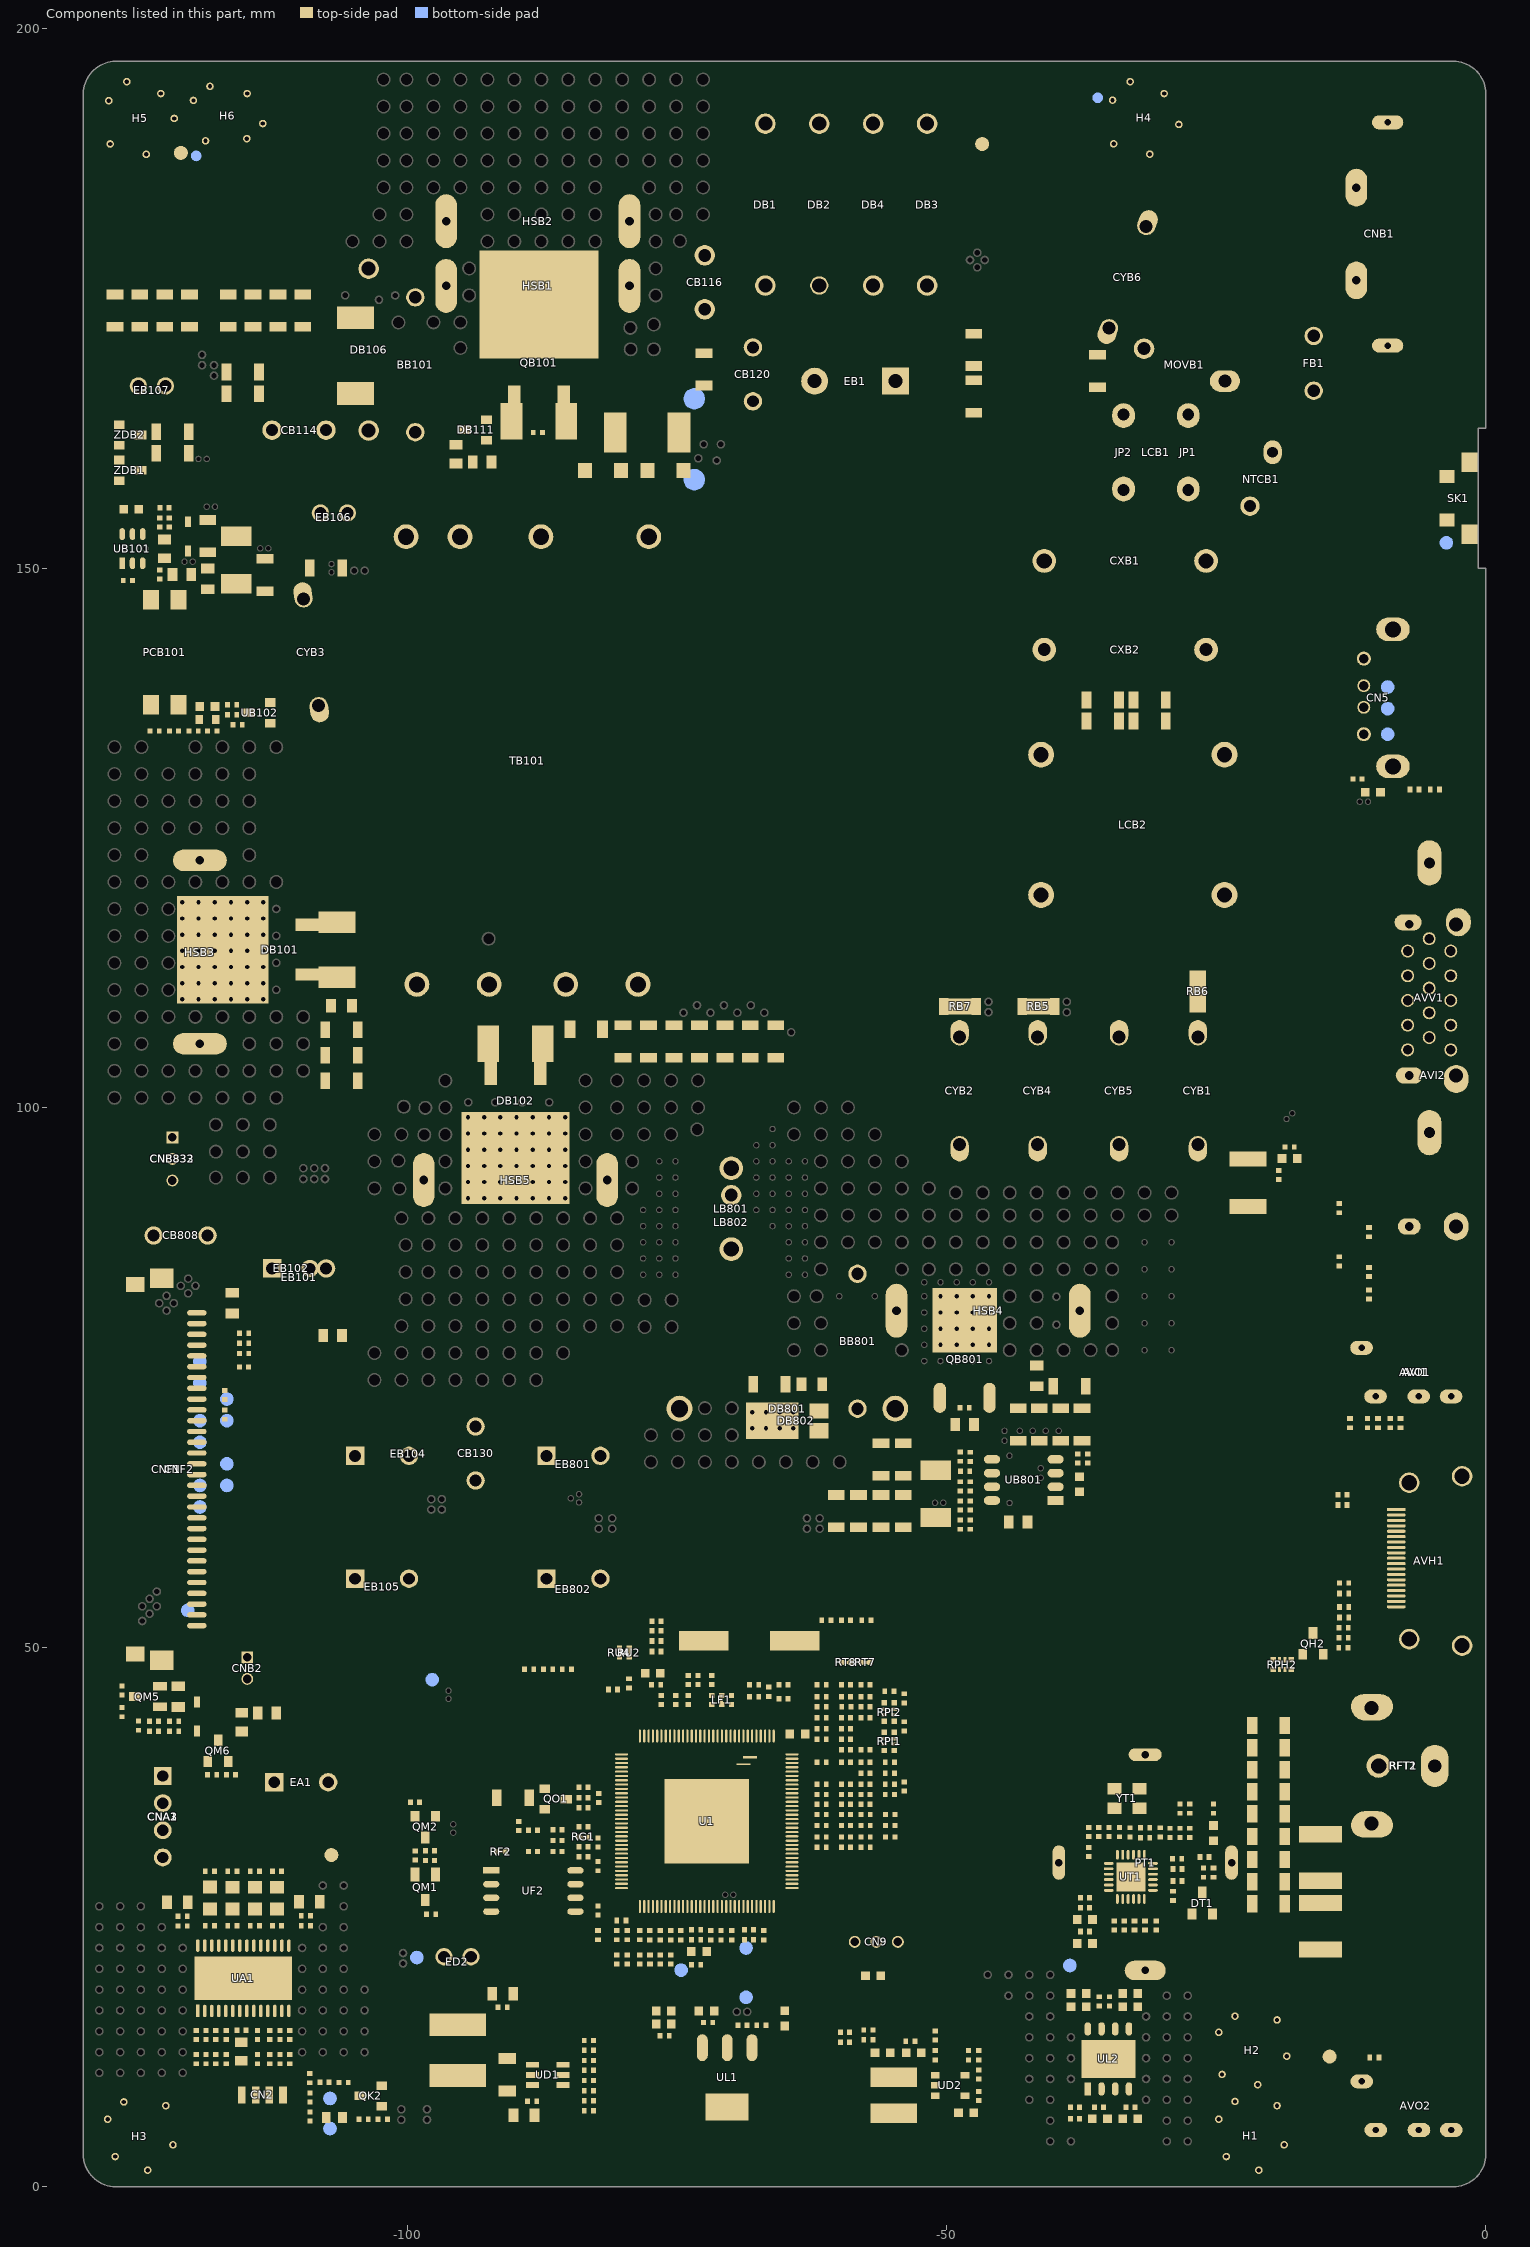
[diagram p0: the components of this part, seen from the top]
# Altium PCB MISC84438.PcbDoc (part 14 of 15)
Units mm, origin at the board's own origin, x right, y up, seen from the top; angles counter-clockwise.
Board outline 130 x 197 mm, 2 copper layers (TopLayer, BottomLayer), stack 1.571 mm thick; 574 components, 314 nets, 2636 pads, 811 vias.

## Other copper
TopLayer:
  drawing of 201 lines, arcs and shapes, not listed
  text "TopLayer" at 176.584,29.998 h1.52
  text ".GTL" at 186.985,29.889 h1.52
BottomLayer:
  rectangle net GND: -121.006,187.35 -118.212,189.408
  rectangle net GND: -48.768,41.034 -48.539,41.669
  rectangle net GND: -7.645,96.266 -3.2,98.806
  rectangle net GND: -2.54,116.18 -0.965,118.923
  rectangle net GND: -2.75,100.736 -1.219,103
  rectangle net GND: -4.661,117 -2.75,119.418
  rectangle net GND: -10.02,129.451 -7.493,131.496
  rectangle net GND: -7.887,121.539 -3.2,123.952
  rectangle net GND: -4.534,101.994 -0.991,103.746
  rectangle: 172.367,23.897 175.674,25.897
  rectangle net GND: -97.155,42.037 -96.862,46.152
  rectangle net GND: -4.978,116.053 -4.521,116.688
  pour cut-out: -35.8,42.2 -20.9,42.2 -20.8,42.1 -20.8,41.529 -35.129,41.529
  pour cut-out: -90.2,54.291 -90.2,58.3 -88.5,60 -87.9,60 -87.9,56.827 -87.073,56
  region net N-1: -14.6,186.4 -14,187 -12.4,187 -12.4,183.6 -14,183.6 -14.6,184.2
  region net D_QB101: -102.502,196.456 -71.349,196.456 -70.866,195.974 -70.866,177.902 -71.526,177.241 -73.707,177.241 -76.429,174.519 -76.429,167.107 -78.461,165.075 -90.634,165.075 -96.679,171.12 -108.814,171.12 -110.541,172.847 -110.541,176.835 -102.819,184.556 -102.819,196.139
  region net VBL: -72.278,93.858 -72.278,95.601 -68.224,99.654 -68.224,103.49 -68.458,103.723 -72.024,103.723 -72.791,104.491 -74.066,104.491 -74.066,95.113 -72.659,93.706 -72.507,93.858
  region net GND: 213 vertices and 0 holes, not listed, extent -60.377,22.169 -58.5,23.205
  region net GND: -31.6,181.1 -32.3,181.8 -32.3,184.928 -36.855,189.484 -36.855,191.145 -36.4,191.6 -33.7,188.9 -29.7,188.9 -27.7,190.9 -27.7,191 -27.006,190.306 -27.006,185.394 -31.3,181.1
  region net GND: -106.586,99.586 -107.4,100.4 -108.6,100.4 -111,98 -111,93.3 -110.7,93 -107.4,93 -107.2,93.2 -107.2,96.2 -105.3,98.1 -105.3,99.1 -105.661,99.1 -106.366,99.805
  region net L: -27.544,123.232 -27.376,123.4 -23.245,123.4 -23.078,123.232 -23.078,119.522 -24,118.6 -25,118.6 -27.544,121.144
  region net N: -42.4,120.8 -43.3,121.7 -43.3,122.4 -43.2,122.4 -42.3,123.3 -37.969,123.3 -37.901,123.232 -37.901,121.039 -40.439,118.5 -42,118.5 -42.4,118.9
  region net N-1: -36.496,162.91 -36.496,165.204 -32.5,169.2 -32.5,170.6 -32,171.1 -29.8,171.1 -29.3,170.6 -29.3,169.3 -32.03,166.57 -32.03,162.91 -32.139,162.8 -36.386,162.8
  region net L-1: -11.3,175.4 -15.9,170.8 -16.3,170.8 -18.4,172.9 -18.4,174 -13.9,178.5 -11.9,178.5 -11.3,177.9
  region net GND: -39.218,60.604 -39.929,59.893 -49.327,59.893 -49.86,59.36 -77.673,59.36 -78.753,58.28 -78.753,57.036 -76.073,54.356 -74.473,55.956 -40.919,55.956 -38.786,58.09 -38.786,60.173
  region net GND: -34.9,194.843 -36.195,194.843 -36.855,194.183 -36.855,192.71 -36.017,191.872 -34.722,193.167 -34.722,194.666
  region net LED_FB: -85.154,63.246 -85.154,64.364 -84.951,64.567 -83.859,64.567 -83.656,64.364 -83.656,63.325 -83.735,63.246
  region net GND: -83.058,68.097 -82.398,68.758 -80.772,68.758 -80.213,68.199 -80.213,54.661 -80.442,54.432 -81.839,54.432 -83.058,55.651
  region net LED+: -63.856,74.549 -80.493,74.549 -82.626,72.415 -82.626,70.053 -79.781,70.053 -78.143,68.415 -78.143,61.938 -77.191,60.985 -66.624,60.985 -63.983,63.627 -56.718,63.627 -54.839,65.507 -54.839,67.564 -54.839,68.148 -55.575,68.885 -62.662,68.885 -62.992,69.215 -62.992,73.685
  region net VBL: -92.913,69.596 -90.91,71.599 -96.215,71.599 -96.215,71.501 -94.31,69.596
  region net GND: -39.535,70.726 -39.243,70.434 -39.243,69.063 -39.56,68.745 -50.863,68.745 -51.079,68.529 -51.079,66.345 -53.063,66.345 -53.063,69.34 -51.676,70.726
  region net GND: -39.573,68.402 -48.603,68.402 -48.831,68.174 -48.831,63.792 -49.225,63.398 -51.41,63.399 -51.41,61.366 -51.029,60.985 -40.775,60.985 -39.129,62.632 -39.129,67.958
  region net NetBB801_2: -56.007,74.6 -54.102,72.695 -54.102,71.171 -54.915,70.358 -60.757,70.358 -61.417,71.018 -61.417,73.889 -60.706,74.6
  region net LED+: -87.073,59.004 -86.868,59.004 -86.081,58.217 -86.081,55.245 -86.716,54.61 -87.02,54.61 -87.579,55.169 -87.579,57.99 -87.073,58.496
  region net GND: -51.41,62.941 -51.41,63.551 -51.257,63.703 -50.063,63.703 -49.759,63.398 -49.759,63.144 -49.962,62.941
  region net GND: -53.061,67.437 -53.061,65.329 -55.931,62.459 -63.398,62.459 -63.602,62.255 -63.602,60.63 -63.424,60.452 -55.118,60.452 -51.079,64.491 -51.079,67.437
  region net L-4: -26.38,127.537 -26.962,125.835 -27.513,127.537
  region net L-4: -25.272,127.537 -25.854,125.835 -26.405,127.537
  region net L-4: -23.047,127.537 -23.629,125.835 -24.18,127.537
  region net L-4: -24.164,127.537 -24.746,125.835 -25.297,127.537
  region net L: -26.426,123.232 -25.844,124.935 -25.293,123.232
  region net L: -27.544,123.232 -26.962,124.935 -26.411,123.232
  region net L: -25.319,123.232 -24.736,124.935 -24.186,123.232
  region net L: -24.211,123.232 -23.629,124.935 -23.078,123.232
  region net L-3: -22.5,154.8 -21.222,154.8 -20.803,155.219 -20.803,156.464 -21.387,157.048 -21.387,167.259 -22.428,168.3 -25.1,168.3 -28.911,164.489 -28.911,162.91 -28.801,162.8 -24.8,162.8 -24.444,162.91 -24.444,165.656 -24.2,165.9 -23.6,165.9 -23.419,165.719 -23.419,155.719
  region net L-2: -16.2,167.2 -15.3,166.3 -15.3,163.9 -19.4,159.8 -19.7,159.8 -20.3,160.4 -20.3,163.1
  region net Vbridge: -57.328,169.291 -57.328,167.818 -55.626,166.116 -52.934,166.116 -52.629,166.421 -52.629,171.602 -55.855,174.828 -55.855,178.308 -56.261,178.714 -62.103,178.714 -62.687,178.13 -62.687,174.622 -62.128,174.063 -59.179,174.063 -55.093,169.977 -55.093,168.58 -55.296,168.377 -55.905,168.377 -56.82,169.291
  region net N: -57.683,193.835 -56.675,194.843 -50.698,194.843 -49.835,193.98 -49.835,188.722 -56.998,188.722 -57.683,189.408
  region net L: -67.691,193.827 -67.691,189.408 -61.214,182.931 -59.288,182.931 -59.288,184.993 -60.909,186.614 -60.909,193.878 -61.849,194.818 -66.7,194.818
  region net N: -41.234,123.232 -41.816,124.935 -42.367,123.232
  region net N: -40.126,123.232 -40.709,124.935 -41.259,123.232
  region net N: -37.901,123.232 -38.483,124.935 -39.034,123.232
  region net N: -39.019,123.232 -39.601,124.935 -40.152,123.232
  region net N-2: -41.281,127.537 -40.699,125.835 -40.148,127.537
  region net N-2: -42.398,127.537 -41.816,125.835 -41.265,127.537
  region net N-2: -40.173,127.537 -39.591,125.835 -39.04,127.537
  region net N-2: -39.065,127.537 -38.483,125.835 -37.932,127.537
  region net N-2: -35.331,158.605 -35.914,160.307 -36.465,158.605
  region net N-2: -34.224,158.605 -34.806,160.307 -35.357,158.605
  region net N-2: -31.998,158.605 -32.581,160.307 -33.131,158.605
  region net N-2: -33.116,158.605 -33.698,160.307 -34.249,158.605
  region net N-1: -35.378,162.91 -34.796,161.207 -34.245,162.91
  region net N-1: -36.496,162.91 -35.914,161.207 -35.363,162.91
  region net N-1: -34.27,162.91 -33.688,161.207 -33.137,162.91
  region net N-1: -33.163,162.91 -32.581,161.207 -32.03,162.91
  region net L-4: -25.559,158.605 -24.977,160.307 -24.426,158.605
  region net L-4: -26.666,158.605 -26.084,160.307 -25.533,158.605
  region net L-4: -28.892,158.605 -28.31,160.307 -27.759,158.605
  region net L-4: -27.774,158.605 -27.192,160.307 -26.641,158.605
  region net L-3: -25.562,162.91 -26.144,161.207 -26.695,162.91
  region net L-3: -24.444,162.91 -25.027,161.207 -25.577,162.91
  region net L-3: -26.67,162.91 -27.252,161.207 -27.803,162.91
  region net L-3: -27.778,162.91 -28.36,161.207 -28.911,162.91
  region net NetCB118_2: -74.587,109.918 -66.611,109.918 -63.652,106.959 -63.653,105.511 -64.11,105.054 -71.222,105.054 -72.72,106.553 -74.93,108.763 -74.93,109.576
  region net GND: -108.407,138.024 -107.01,138.024 -104.546,135.56 -104.546,122.784 -97.104,115.341 -97.104,111.328 -101.067,111.328 -101.067,115.646 -107.061,121.641 -107.061,133.909 -108.661,135.509 -109.245,136.093 -109.245,137.592 -108.814,138.024
  region net 12V: -129.337,135.23 -128.143,136.423 -118.948,136.423 -117.196,134.671 -109.347,134.671 -108.077,133.401 -108.077,121.107 -102.311,115.341 -102.311,108.204 -112,98.515 -112,93.2 -112.3,92.9 -119.5,92.9 -120.1,93.5 -120.1,98.4 -121,99.3 -127.646,99.3 -129.337,100.99
  region net NetCB118_1: -86.182,112.573 -84.379,112.573 -83.591,111.785 -83.591,110.338 -83.972,109.957 -86.589,109.957 -86.995,110.363 -86.995,111.76
  region net NetCB117_1: -80.112,110.846 -79.223,109.957 -77.902,109.957 -77.064,110.795 -77.064,113.436 -80.721,117.094 -92.253,117.094 -93.878,115.468 -93.878,110.592 -93.243,109.957 -91.77,109.957 -87.63,114.097 -83.363,114.097
  region net SGND: -62.103,168.567 -65.227,168.567 -66.358,167.437 -67.17,167.437 -74.358,160.249 -74.358,157.632 -73.939,157.213 -71.463,157.213 -70.485,158.191 -70.485,161.607 -66.548,165.544 -64.021,165.544 -62.065,167.5
  region net NetBB101_2: -89.37,154.623 -86.208,154.623 -85.877,154.292 -85.877,152.121 -86.208,151.79 -88.786,151.79 -89.37,152.375
  region net 12V-OVP: -101.067,154.635 -99.314,154.635 -98.628,153.949 -98.628,152.171 -98.996,151.803 -101.067,151.803 -101.536,152.273 -101.536,154.165
  region net Vbridge: -79.197,160.909 -79.908,161.62 -79.4,162.128 -77.038,162.128 -76.581,161.671 -76.581,154.508 -76.06,153.987 -76.06,152.273 -76.517,151.816 -78.816,151.816 -79.197,152.197
  region net NetCB114_2: -103.048,165.278 -107.594,165.278 -108.382,164.49 -108.382,161.595 -107.747,160.96 -103.048,160.96 -102.514,161.493 -102.514,164.744
  region net Vbridge: -119.253,170.256 -118.643,170.256 -117.145,168.758 -117.145,167.691 -117.399,167.437 -118.237,167.437 -119.482,168.681 -119.482,170.028
  region net D_QB801: -29.312,93.218 -27.771,91.677 -27.771,74.769 -30.251,72.288 -51.003,72.288 -54.559,75.844 -64.414,75.844 -65.532,76.962 -65.532,86.589 -68.707,89.764 -69.723,89.764 -71.013,91.054 -71.013,94.894 -64.066,101.841 -58.623,101.841 -50,93.218
  region net VBL: -72.187,93.369 -72.187,80.955 -74.427,78.715 -81.686,78.715 -82.093,79.121 -82.093,89.764 -78.074,93.783
  region net VBL: -71.049,80.564 -75.171,76.441 -74.778,76.048 -68.047,76.048 -67.259,76.835 -67.259,85.877 -69.393,88.011 -70.46,88.011 -71.049,87.422
  region net SGND: -123.114,167.132 -123.114,164.389 -122.758,164.033 -122.631,164.16 -121.945,164.16 -121.945,165.252 -121.869,165.329 -121.315,165.329 -121.115,165.528 -122.718,167.132
  region net NetBB101_2: -97.255,161.669 -97.255,163.066 -99.012,164.824 -99.429,164.824 -99.429,163.31 -97.993,161.874
  pour cut-out: -119.969,76.5 -119.969,74.599 -119.385,74.016 -119.283,74.117 -119.283,76.886
  pour cut-out: -115.958,72.801 -115.958,70.991 -116.438,70.51 -116.7,70.772 -116.7,73
  pour cut-out: -119.942,70.801 -119.942,69.138 -119.359,68.555 -119.2,68.714 -119.2,71
  pour cut-out: -115.958,66.801 -115.958,65.175 -116.337,64.795 -116.7,65.159 -116.7,67
  pour cut-out: -119.942,64.801 -119.942,63.118 -119.537,62.713 -119.2,63.05 -119.2,65
  pour cut-out: -42.253,58.369 -36.354,64.268 -37.454,65.367 -37.91,64.911 -37.91,63.851 -41.08,60.681 -45.822,60.681 -47.053,59.449 -45.974,58.369
  pour cut-out: -2.688,157.65 -2.688,155.35 -2.617,155.421 -1.826,155.421 -1.826,157.534 -1.816,157.543
  region net 5V_USB: -11.824,128.689 -12.014,128.499 -12.014,127.749 -11.735,127.47 -11.011,127.47 -10.604,127.876 -10.604,128.486 -10.808,128.689
  pour cut-out: -87.41,50.834 -84.626,53.619 -79.807,53.619 -78.753,54.673 -78.753,59.512 -76.695,61.57 -76.695,66.015 -82.588,66.015 -83.414,66.84 -88.036,62.217 -88.036,51.46
  pour cut-out: -115.073,85.522 -129.54,85.522 -130.404,84.658 -131.229,85.484 -131.229,88.824 -113.474,88.824 -113.474,86.208 -114.605,85.077 -114.628,85.077
  region net 12V: -120.879,84.557 -123.393,82.042 -123.393,81.686 -122.466,80.759 -121.755,80.759 -119.189,83.325 -119.189,83.655 -120.091,84.557
  region net 1.15V_STB: -70.663,27.356 -70.815,27.203 -70.815,26.911 -70.168,26.264 -69.647,26.264 -69.367,26.543 -69.367,27.14 -69.583,27.356
  region net 1.15V_STB: -69.38,17.272 -68.948,17.272 -68.047,16.37 -68.047,16.027 -68.288,15.786 -69.647,15.786 -69.85,15.989 -69.85,16.37 -69.583,16.637 -69.583,17.069
  region net 12V: -97.904,7.569 -100.711,7.569 -100.914,7.366 -100.914,6.007 -100.698,5.791 -97.866,5.791 -97.625,6.032 -97.625,7.29
  region net 5V_STB: -98.87,21.653 -99.085,21.869 -99.936,21.869 -100.127,22.06 -100.546,22.06 -100.774,21.831 -100.774,20.511 -100.546,20.282 -100.178,20.282 -99.86,20.599 -99.187,20.599 -98.87,20.917
  region net GND: -2.908,103.653 -2.908,103 -1.661,103 -1.13,103.53 -1.13,104.407 -1.283,104.559 -2.002,104.559
  region net 12V: -123.571,55.575 -124.968,54.178 -124.968,51.956 -114.148,41.135 -114.148,37.77 -113.081,36.703 -111.811,36.703 -111.43,37.084 -111.43,41.834 -114.745,45.148 -114.745,47.282 -114.986,47.523 -116.205,47.523 -122.758,54.077 -122.758,55.321 -123.012,55.575
  region net SGND: -108.102,157.632 -98.374,157.632 -94.385,153.643 -95.629,152.398 -98.984,155.753 -102.768,155.753 -104.445,154.076 -104.445,153.746 -104.753,153.438 -105.838,153.438 -106.1,153.7 -106.1,155.4 -108.102,157.402
  region net SGND: -103.632,151.359 -101.981,149.708 -101.981,147.955 -102.083,147.853 -102.083,147.752 -102.133,147.701 -103.124,147.701 -105.207,149.784 -105.207,150.901 -104.75,151.359
  region net GND: -23.673,97.384 -18.313,92.025 -22.345,87.993 -28.585,94.234 -49.034,94.234 -49.86,95.06 -49.86,96.825 -49.301,97.384
  region net N-2: -32.093,158.7 -31.998,158.605 -31.998,157.202 -32.8,156.4 -34.8,156.4 -36.465,158.065 -36.465,158.605 -36.37,158.7
  region net L-4: -24.52,158.7 -24.426,158.605 -24.426,157.774 -25.8,156.4 -27.9,156.4 -28.892,157.392 -28.892,158.605 -28.797,158.7
  region: -11,190.7 -11.4,191.1 -11.4,192.4 -11,192.8 -8.5,192.8 -7.9,192.2 -7.9,191.2 -8.4,190.7
  region net SGND: -103.632,151.359 -107.041,151.359 -107.4,151 -107.4,149.5 -107.2,149.3 -103.492,149.3 -103.2,149.592 -103.2,150.927
  pour cut-out: -14.682,116.139 -12.217,118.604 -12.217,123.2 -12.5,123.2 -12.8,123.5 -16.2,120.1 -16.8,120.1
  region net L-4: -23.047,127.537 -23.047,132.249 ccw(c-24.627,132.249) -23.51,133.367 -23.753,133.367 ccw(c-23.753,130.827) -25.549,132.623 -28.971,129.201 -28.971,127.322 -23.262,127.322
  region net VBL: -95.5,108.382 -76.683,108.382 -72.187,103.886 -72.187,92.71 -74.727,90.17 -79.121,90.17 ccw(c-79.121,88.824) -80.467,88.824 -80.467,79.68 -87.046,73.101 -101.549,73.101 -104.14,70.51 -104.14,55.778 -104.419,55.499 -105.639,55.499 -106.68,56.54 -106.68,75.32 -100.8,81.2 -100.8,87.2 -106.2,92.6 -106.2,95.628 -95.5,106.328
  region net N-2: -42.398,127.537 -42.398,132.249 cw(c-40.818,132.249) -41.935,133.367 -41.692,133.367 cw(c-41.692,130.827) -39.896,132.623 -36.474,129.201 -36.474,127.322 -42.183,127.322
  pour cut-out: -7.966,6.576 -8.071,6.471 ccw(c-7.219,5.619) -8.424,5.619 cw(c-8.424,6.391) -8.971,5.845 -9.8,6.674 ccw(c-10.417,7.291) -9.545,7.291 -9.545,7.328 ccw(c-9.545,8.204) -8.925,7.585 -8.865,7.645 -8.66,7.441 ccw(c-8.357,7.744) -8.357,7.315
  pour cut-out: -2.003,158.335 -1.726,158.612 ccw(c-2.917,159.804) -1.232,159.804 -1.232,152.379 cw(c-1.239,152.379) -1.234,152.375 -1.234,153.896 ccw(c-2.003,153.896) -2.003,154.665 ccw(c-2.003,154.842) -1.826,154.842 -1.826,156.011 ccw(c-1.826,156.603) -1.234,156.603 -1.234,156.965 -2.003,156.965
  pour cut-out: -2.034,6.576 -0.746,5.289 cw(c-1.267,4.768) -0.531,4.768 cw(c0.38,4.768) -0.264,5.413 0,5.677 -0.305,5.982 cw(c1.104,7.391) -0.889,7.391
  pour cut-out: -1.5,8.567 -1.211,8.856 ccw(c-2.909,10.554) -0.508,10.554 -0.508,8.479 cw(c-0.586,8.479) -0.531,8.424 cw(c-1.461,9.354) -1.461,8.039 -1.499,8.039
  pour cut-out: -10.451,141.108 -9.041,141.108 cw(c-9.041,139.535) -7.468,139.535 -7.468,134.607 cw(c-8.928,134.607) -8.928,133.147 -11.231,133.147 cw(c-11.231,134.937) -13.022,134.937 -13.022,138.697 cw(c-10.601,138.697) -10.601,141.118
  pour cut-out: -9.552,75.776 -9.552,75.743 -10.622,74.674 -9.197,73.25 -8.397,73.25 -8.397,73.588 cw(c-7,73.588) -7.988,74.576 cw(c-7.466,75.098) -8.204,75.098 -8.204,75.603
  text ".GBL" at 186.977,24.448 h1.52
  text "BottomLayer" at 176.248,24.41 h1.52
MultiLayer:
  pour cut-out: -16.993,45.822 -19.736,45.822 -21.101,44.457 -21.101,41.974 -20.714,41.974 -18.872,43.815 -16.967,43.815 -16.434,44.348 -16.434,45.263

## Silkscreen, mask and mechanical layers (free items; w line width, h text height)
TopOverlay:
  drawing of 620 lines, arcs and shapes, not listed
  text "AC IN" at -19.304,180.213 h1.52
  text "Solder Mask:" at 168.941,155.426 h1.52
  text "IPC SM-840" at 179.418,155.401 h1.52
  text "Silkscreen Color:" at 198.875,155.401 h1.52
  text "White" at 211.041,155.401 h1.52
  text "Units:" at 198.875,152.886 h1.52
  text "PTH Copper Thickness:" at 168.941,152.861 h1.52
  text ">20um" at 186.048,152.835 h1.52
  text "mm" at 203.904,152.848 h1.52
  text "Dielectric Constant Er@1GHz To 1MHz:" at 168.932,150.347 h1.52
  text "4.2 --- 4.6" at 198.891,150.36 h1.52
  text "Panel Size:" at 168.89,147.844 h1.52
  text "2L,2,130.00×197.00mm,FR4(TG130-CTI175),1OZ,Green,OSP,1.6mm" at 176.641,147.845 h1.52
  text "Silkscreen on PTH:" at 168.903,145.266 h1.52
  text "Primary Side Retained;" at 182.06,145.241 h1.52
  text "Secondary Side  Removed for Soldering" at 198.875,145.203 h1.52
  text "Special Requirements" at 168.877,142.963 h1.52
  text "If engineering questions are not answered within 2 hours, contact the engineering team" at 216.798,142.778 h1.52
  text "UL requires special handling; see special notes in the attachment" at 184.227,142.748 h1.52
  text "1. Lead-free HASL (HAL_LF, Lead Free Hot Air Leveling)" at 183.885,140.332 h1.52
  text "2. Organic solderability preservative (OSP, Organic Solderability Preservatives)" at 183.885,138.198 h1.52
  text "3. Electroless nickel immersion gold (ENIG, Electroless Nickel/Immersion Gold)" at 183.847,135.874 h1.52
  text "Plated Technics" at 170.782,134.992 h1.52
  text "4. ENIG + gold finger (ENIG_G/F, Electroless Nickel/Immersion Gold + Gold Finger)" at 183.885,133.829 h1.52
  text "5. Gold plating (Gold_plated, Gold-plated)" at 183.911,131.785 h1.52
  text "6. Gold plating + gold finger (Gold_Plated_G/F, Gold-plated + Gold Finger)" at 183.924,129.803 h1.52
  text "Impedance Control" at 168.997,123.997 h1.52
  text "Target Impedance" at 189.237,124 h1.52
  text "Layer(s)" at 227.696,124.002 h1.52
  text "Width & Clearance" at 208.181,123.994 h1.52
  text "75 +/- 10% Ohm" at 189.801,121.442 h1.52
  text "G/12/15.8/12/G mil" at 207.099,121.425 h1.52
  text "layer 1" at 227.696,121.428 h1.52
  text "Single End Impedance" at 168.997,120.268 h1.52
  text "75 +/- 10% Ohm" at 189.801,118.953 h1.52
  text "G/6.2/7.1/6.2/G mil" at 207.099,118.935 h1.52
  text "layer 1" at 227.696,118.939 h1.52
  text "[ Zo ]" at 174.674,116.782 h1.52
  text "2" at -254.691,113.421 h4.06 r180
  text "G/5/7/5/7/5/G mil" at 207.353,111.493 h1.52
  text "100 +/- 10% Ohm" at 189.471,111.468 h1.52
  text "layer 1" at 227.975,111.422 h1.52
  text "Differential Impedance" at 168.994,110.068 h1.52
  text "[ Zo ]" at 174.661,106.935 h1.52
  text "( G: Ground )" at 172.377,104.205 h1.52
  text "90 +/- 10% Ohm" at 190.132,103.899 h1.52
  text "layer 1" at 227.874,103.879 h1.52
  text "G/5/11/5/11/5/G mil" at 207.353,103.81 h1.52
  text "Common Mode Impedance" at 168.48,98.574 h1.52
  text "[ Zc ]" at 174.779,96.517 h1.52
  text "LED DRIVER" at -117.8,91.4 h1.52
  text "Refer to Gerber documents GTP&GBP for Stencil aperture design" at 191.723,89.806 h1.52
  text "Stencil (Stencil)" at 168.843,87.342 h1.52
  text "New" at 191.713,84.902 h1.52
  text "1" at -5.309,83.579 h4.06
  text "Test jig (Testing jig)" at 168.795,82.373 h1.52
  text "The same as XXXXXXXXXXXXXXX XXXXXX" at 191.713,82.355 h1.52
  text "Wave-soldering jig (Wave-soldering jig)" at 168.851,79.877 h1.52
  text "New" at 191.713,79.813 h1.52
  text "Solder paste" at 191.66,77.292 h1.52
  text "Production process" at 168.812,77.254 h1.52
  text "[Process and notes]" at 173.39,75.099 h1.52
  text "Special requirements (Special Requirements)" at 168.838,72.225 h1.52
  text "SMD parts over 2mm high on the wave-solder side" at 168.83,69.651 h1.52
  text "Packaging notes (Package Attention)" at 168.822,67.207 h1.52
  text "[Easily damaged parts]" at 174.952,65.054 h1.52
  text "LVDS" at -117.272,63.83 h1.52
  text "JX Label" at -26.847,62.939 h2.03 r90
  text "New footprint matching (Footprint Matching)" at 168.822,62.127 h1.52
  text "[New component footprint]" at 174.596,59.999 h1.52
  text "(Automated Testing Support)" at 176.908,57.091 h1.14
  text "Automated test support" at 168.818,57.002 h1.52
  text "XXXXXX" at -71.641,55.766 h3.05
  text "Yes" at 191.64,55.579 h1.52
  text "[Reserve suction-nozzle and press-bar positions]" at 172.894,54.856 h1.52
  text "V3 2018.12.08" at -71.641,53.34 h3.05
  text "PWR UPGRADE" at -117.526,52.654 h1.27
  text "GND" at -112.573,48.59 h1.27
  text "12V" at -112.598,46.482 h1.27
  text "Layer Stack Up Detail for" at 172.402,45.724 h2.54
  text ".Pcb_File_Name_No_Path" at 199.347,45.724 h2.54
  text "Layer" at 176.576,41.971 h1.27
  text "Gerber" at 186.018,41.971 h1.27
  text "Layer" at 193.921,41.971 h1.27
  text "Layer" at 210.082,41.971 h1.27
  text "Copper" at 230.12,41.971 h1.27
  text "Dielectric" at 238.039,41.971 h1.27
  text "Stack up" at 210.082,40.679 h1.27
  text "Height" at 238.039,40.679 h1.27
  text "Name" at 176.576,40.641 h1.27
  text "Document" at 186.018,40.641 h1.27
  text "Ordor" at 193.921,40.641 h1.27
  text "Thickness" at 230.12,40.641 h1.27
  text "TopOverlay" at 176.569,34.726 h1.52
  text ".GTO" at 186.972,34.661 h1.52
  text "0.4mil" at 237.971,32.502 h1.52
  text "1" at 195.272,29.882 h1.52
  text "1.4mil" at 230.451,29.88 h1.52
  text "2" at 195.274,24.47 h1.52
  text "1.4mil" at 230.408,24.445 h1.52
  text "0.4mil" at 238.039,22.04 h1.52
  text "DEBUG" at -49.8,20.4 h1.52 r90
  text "IR" at -119.482,8.788 h1.27
  text "Notes:" at 168.234,7.743 h2.03
  text "LED" at -108.026,7.595 h1.27
  text "1. No Plated Through Hole  overlap each other should be combined ,Residues between them should be eliminated." at 168.212,5.51 h1.52
  text "2. Plated Through Hole superposition should be made as a bigger one." at 168.211,3.577 h1.52
  text "3. When there is not enough space for UL authentication marking,Manufacturer ID code and the Bar Code frame," at 168.212,1.837 h1.52
  text "only the Manufacturer  ID code is needed and layed wherever it can be." at 169.695,0.042 h1.52
  text "4. Spacing between two pads of IC package should be covered with solder oil." at 168.212,-1.909 h1.52
  text "5. All trace should be covered with green oil unless otherwise specified. If discovers unusually, please confirm with us." at 168.212,-3.773 h1.52
  text "6. Silkscreen overlaped SMD pads should be removed directly." at 168.212,-5.635 h1.52
  text "7. The width of Carbon Sprayed must be 16mil wider than its trace." at 168.212,-7.44 h1.52
  text "8. Bridging Thickness of V-cut  should be kept within 0.3±0.1mm when the width of single piece bare board is smaller than 20mm." at 168.212,-9.33 h1.52
  text "9. There is no need to plugged with green oil when the diameter of vias is bigger than 0.6mm." at 168.212,-11.409 h1.52
  text "10. All vias under BGA must be covered and plugged with Solder oil." at 168.212,-13.437 h1.52